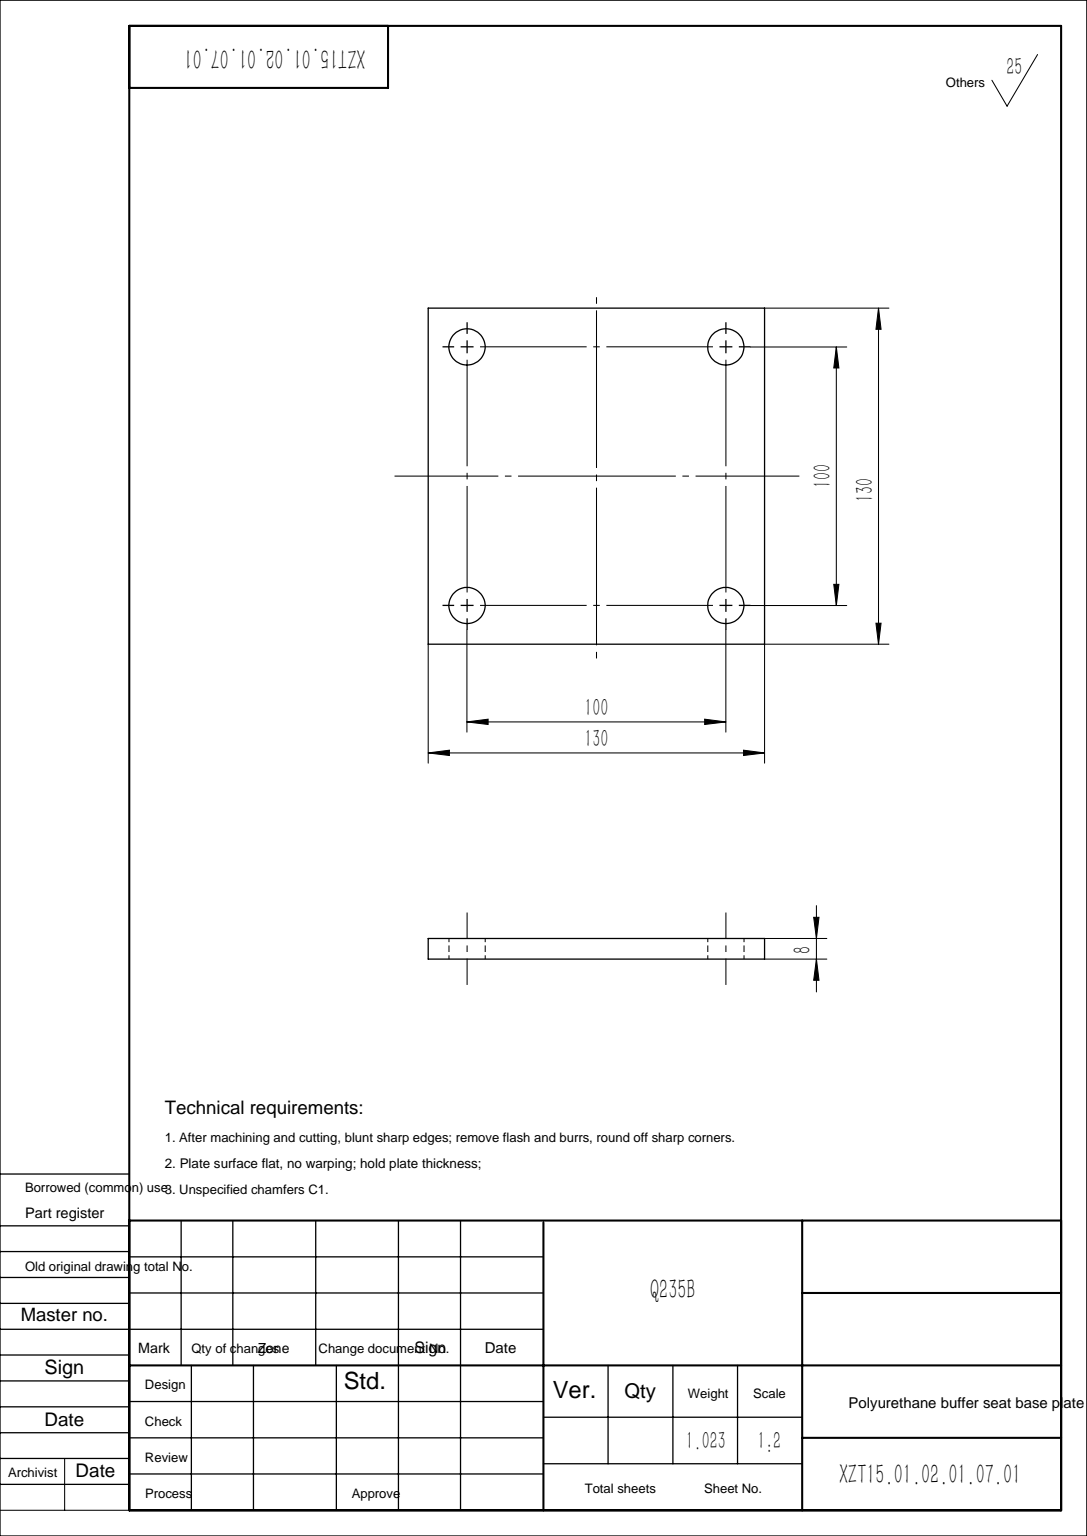
SolidWorks part; units mm, degrees
material "Q235B"
ref_plane "Front Plane" through (0, 0, 0) normal (0, 0, 1) x (1, 0, 0)
ref_plane "Top Plane" through (0, 0, 0) normal (0, 1, 0) x (1, 0, 0)
ref_plane "Right Plane" through (0, 0, 0) normal (1, 0, 0) x (0, 0, -1)
sketch "Sketch1" plane through (0, 0, 0) normal (0, 1, 0) x (1, 0, 0)
  line L1 (65, -65) -> (-65, -65)
  line L2 (65, -65) -> (65, 65)
  line L3 (65, 65) -> (-65, 65)
  line L4 (-65, -65) -> (-65, 65)
  line L5 (65, -65) -> (-65, 65) construction
  line L6 (65, 65) -> (-65, -65) construction
  point P0 (0, 0)
  dimension "D1" = 130
  dimension "D2" = 130
extrude "Boss-Extrude1" add sketch "Sketch1" along normal blind 8
hole_wizard "Ø14.0 (14) Diameter Hole1" positions "Sketch2" profile "Sketch3" hole size "Ø14.0" standard "GB" end condition up to next
sketch "Sketch2" plane through (0, 8, 0) normal (0, 1, 0) x (1, 0, 0)
  line L0 (-50, -50) -> (50, -50) construction
  line L1 (-50, -50) -> (-50, 50) construction
  line L2 (0, 0) -> (0, -50) construction
  line L4 (0, 0) -> (-50, 0) construction
  point P0 (-50, -50)
  point P8 (50, -50)
  point P9 (50, 50)
  point P10 (-50, 50)
  dimension "D3" = 90
  dimension "D4" = 100
  dimension "D5" = 100
  dimension "D1" = 2
  dimension "D2" = 2
sketch "Sketch3" plane through (-50, 8, 50) normal (1, 0, 0) x (0, 0, 1)
  line L0 (0, 0) -> (0, 8)
  line L1 (0, 8) -> (7, 8)
  line L2 (7, 8) -> (7, 0)
  line L5 (7, 0) -> (0, 0)
  line L11 (0, -6.35) -> (0, 107.95) construction
  dimension "通孔孔直径" = 14
  dimension "通孔孔深度" = 8
chamfer "Chamfer1" [suppressed] distance 10 angle 45
fillet "Fillet1" [suppressed] radius 10
